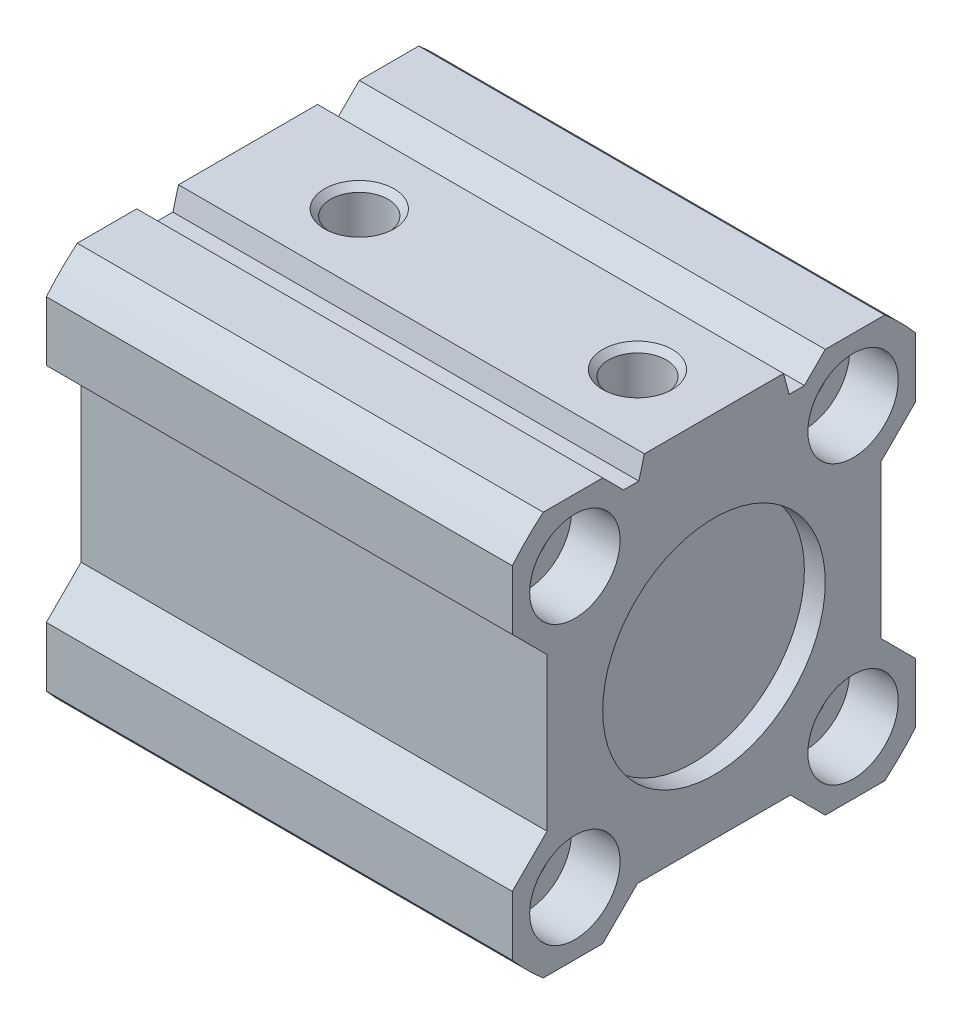
from build123d import *

# Parameters (mm, degrees)
BOSS_EXTRUDE1_DEPTH  = 33.5
HOLE1_D              = 16
HOLE1_DEPTH          = 1.5
SKETCH4_R            = 8
SKETCH4_R_2          = 5.5
CUT_EXTRUDE1_DEPTH   = 5
HOLE2_D              = 4.134
HOLE2_DEPTH          = 6
HOLE2_CSINK_D        = 5
HOLE2_CSINK_ANGLE    = 90
LPATTERN1_COUNT      = 2
LPATTERN1_PITCH      = 20
LPATTERN2_COUNT      = 2
LPATTERN2_PITCH      = 20
LPATTERN2_COUNT_DIR2 = 2
LPATTERN2_PITCH_DIR2 = 20


with BuildPart() as part:
    # Sketch1 → Boss-Extrude1 (new body)
    with BuildSketch(Plane(origin=(0, 0, 0), x_dir=(0, 0, -1), z_dir=(1, 0, 0))):
        with BuildLine():
            Line((-12.278029158, -14.5), (-8, -14.5))
            Line((-8, -14.5), (-5.5, -12))
            Line((-5.5, -12), (5.5, -12))
            Line((5.5, -12), (8, -14.5))
            Line((8, -14.5), (12.278029158, -14.5))
            ThreePointArc((12.278029158, -14.5), (13.435028843, -13.435028843), (14.5, -12.278029158))
            Line((14.5, -12.278029158), (14.5, -8))
            Line((14.5, -8), (12, -5.5))
            Line((12, -5.5), (12, 5.5))
            Line((12, 5.5), (14.5, 8))
            Line((14.5, 8), (14.5, 12.278029158))
            ThreePointArc((14.5, 12.278029158), (13.435028843, 13.435028843), (12.278029158, 14.5))
            Line((12.278029158, 14.5), (8, 14.5))
            Line((8, 14.5), (6.5, 13))
            Line((6.5, 13), (5.401923789, 13))
            Line((5.401923789, 13), (5, 14.5))
            Line((5, 14.5), (-5, 14.5))
            Line((-5, 14.5), (-5.401923789, 13))
            Line((-5.401923789, 13), (-6.5, 13))
            Line((-6.5, 13), (-8, 14.5))
            Line((-8, 14.5), (-12.278029158, 14.5))
            ThreePointArc((-12.278029158, 14.5), (-13.435028843, 13.435028843), (-14.5, 12.278029158))
            Line((-14.5, 12.278029158), (-14.5, 8))
            Line((-14.5, 8), (-12, 5.5))
            Line((-12, 5.5), (-12, -5.5))
            Line((-12, -5.5), (-14.5, -8))
            Line((-14.5, -8), (-14.5, -12.278029158))
            ThreePointArc((-14.5, -12.278029158), (-13.435028843, -13.435028843), (-12.278029158, -14.5))
        make_face()
    extrude(amount=BOSS_EXTRUDE1_DEPTH)

    # Hole1
    with Locations(Plane(origin=(33.5, 0, 0), x_dir=(0, 0, -1), z_dir=(1, 0, 0))):
        with Locations((0, 0)):
            Hole(HOLE1_D / 2, depth=HOLE1_DEPTH)

    # Sketch4 → Cut-Extrude1 (cut)
    with BuildSketch(Plane(origin=(0, 0, 0), x_dir=(0, 0, -1), z_dir=(1, 0, 0))):
        Circle(SKETCH4_R)
        Circle(SKETCH4_R_2, mode=Mode.SUBTRACT)
    extrude(amount=CUT_EXTRUDE1_DEPTH, mode=Mode.SUBTRACT)

    # Sketch5 → Cut-Revolve1 (revolve, cut)
    with BuildSketch(Plane.XY, mode=Mode.PRIVATE) as cut_revolve1_sk:
        Polygon((0, 0), (0, 4), (10, 4), (10, 8), (30, 8), (30, 0), align=None)
    revolve(cut_revolve1_sk.sketch.rotate(Axis((30, 0, 0), (-1, 0, 0)), 270), axis=Axis((30, 0, 0), (-1, 0, 0)), mode=Mode.SUBTRACT)

    # Hole2
    with Locations(Plane(origin=(0, 14.5, 0), x_dir=(1, 0, 0), z_dir=(0, 1, 0))):
        with Locations((8, 0)):
            hole2 = CounterSinkHole(HOLE2_D / 2, HOLE2_CSINK_D / 2, depth=HOLE2_DEPTH, counter_sink_angle=HOLE2_CSINK_ANGLE)

    # LPattern1: Hole2 ×2
    with Locations(*[(i * LPATTERN1_PITCH, 0, 0) for i in range(1, LPATTERN1_COUNT)]):
        add(hole2, mode=Mode.SUBTRACT)

    # Sketch9 → Cut-Revolve2 (revolve, cut)
    with BuildSketch(Plane.XY.offset(10), mode=Mode.PRIVATE) as cut_revolve2_sk:
        Polygon((0, 10), (0, 13.25), (3.5, 13.25), (3.5, 11.75), (30, 11.75), (30, 13.25), (33.5, 13.25), (33.5, 10), align=None)
    cut_revolve2 = revolve(cut_revolve2_sk.sketch.rotate(Axis((33.5, 10, 10), (-1, 0, 0)), 270), axis=Axis((33.5, 10, 10), (-1, 0, 0)), mode=Mode.SUBTRACT)

    # LPattern2: Cut-Revolve2 2 × 2
    with Locations(*[(0, -j * LPATTERN2_PITCH_DIR2, -i * LPATTERN2_PITCH) for i in range(LPATTERN2_COUNT) for j in range(LPATTERN2_COUNT_DIR2) if (i, j) != (0, 0)]):
        add(cut_revolve2, mode=Mode.SUBTRACT)


solid = part.part
